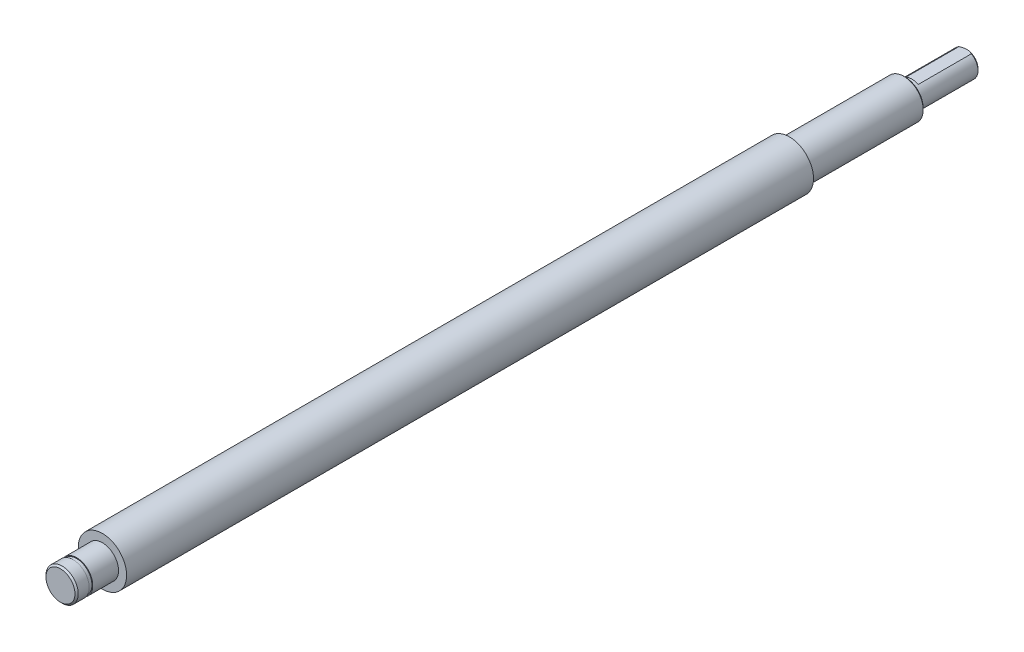
from build123d import *

# Parameters (mm, degrees)
SKETCH_1_R          = 7.5
EXTRUDE_1_DEPTH     = 281
SKETCH_3_W          = 48.87377388
SKETCH_3_H          = 13
SKETCH_4_W          = 35.83639091
SKETCH_4_H          = 82.680612398
SKETCH_8_W          = 33.14878911
SKETCH_8_H          = 39.753572134
CHAMFER_2_SIZE      = 0.5
SKETCH_15_W         = 15.290885205
SKETCH_15_H         = 1.1
CHAMFER_3_SIZE      = 0.5
SKETCH_16_W         = 27.071895425
SKETCH_16_H         = 14.859010271
CUT_EXTRUDE_1_DEPTH = 17


with BuildPart() as part:
    # 草图1 → 凸台-拉伸1 (new body)
    with BuildSketch(Plane.XY):
        Circle(SKETCH_1_R)
    extrude(amount=EXTRUDE_1_DEPTH)

    # 草图3 → 切除-旋转1 (revolve, cut)
    with BuildSketch(Plane(origin=(0, 0, 0), x_dir=(1, 0, 0), z_dir=(0, 1, 0)), mode=Mode.PRIVATE) as cut_revolve_1_sk:
        with Locations((-29.43688694, -274.5)):
            Rectangle(SKETCH_3_W, SKETCH_3_H)
    revolve(cut_revolve_1_sk.sketch.rotate(Axis((0, 0, 281), (0, 0, -1)), 180), axis=Axis((0, 0, 281), (0, 0, -1)), mode=Mode.SUBTRACT)

    # 草图4 → 切除-旋转2 (revolve, cut)
    with BuildSketch(Plane(origin=(0, 0, 0), x_dir=(1, 0, 0), z_dir=(0, 1, 0))):
        with Locations((23.918195455, -13.659693801)):
            Rectangle(SKETCH_4_W, SKETCH_4_H)
    revolve(axis=Axis((0, 0, 281), (0, 0, -1)), mode=Mode.SUBTRACT)

    # 草图8 → 切除-旋转5 (revolve, cut)
    with BuildSketch(Plane(origin=(0, 0, 0), x_dir=(1, 0, 0), z_dir=(0, 1, 0)), mode=Mode.PRIVATE) as cut_revolve_5_sk:
        with Locations((-20.574394555, 0.876786067)):
            Rectangle(SKETCH_8_W, SKETCH_8_H)
    revolve(cut_revolve_5_sk.sketch.rotate(Axis((0, 0, 268), (0, 0, 1)), 180), axis=Axis((0, 0, 268), (0, 0, 1)), mode=Mode.SUBTRACT)

    # 倒角2
    chamfer_2_edges = [part.edges().sort_by_distance(p)[0] for p in [
        (-6, 0, 19),
        (-4, 0, 0),
    ]]
    chamfer(chamfer_2_edges, length=CHAMFER_2_SIZE)

    # 草图15 → 切除-旋转7 (revolve, cut)
    with BuildSketch(Plane(origin=(0, 0, 0), x_dir=(1, 0, 0), z_dir=(0, 1, 0)), mode=Mode.PRIVATE) as cut_revolve_7_sk:
        with Locations((-12.395442603, -276.55)):
            Rectangle(SKETCH_15_W, SKETCH_15_H)
    revolve(cut_revolve_7_sk.sketch.rotate(Axis((0, 0, 281), (0, 0, 1)), 180), axis=Axis((0, 0, 281), (0, 0, 1)), mode=Mode.SUBTRACT)

    # 倒角3
    chamfer_3_edges = [part.edges().sort_by_distance(p)[0] for p in [
        (-5, 0, 281),
    ]]
    chamfer(chamfer_3_edges, length=CHAMFER_3_SIZE)

    # 草图16 → 切除-拉伸1 (cut)
    with BuildSketch(Plane(origin=(0, 0, 0), x_dir=(-1, 0, 0), z_dir=(0, 0, -1))):
        with Locations((-4.49502023, 10.929505136)):
            Rectangle(SKETCH_16_W, SKETCH_16_H)
    extrude(amount=-CUT_EXTRUDE_1_DEPTH, mode=Mode.SUBTRACT)


solid = part.part
